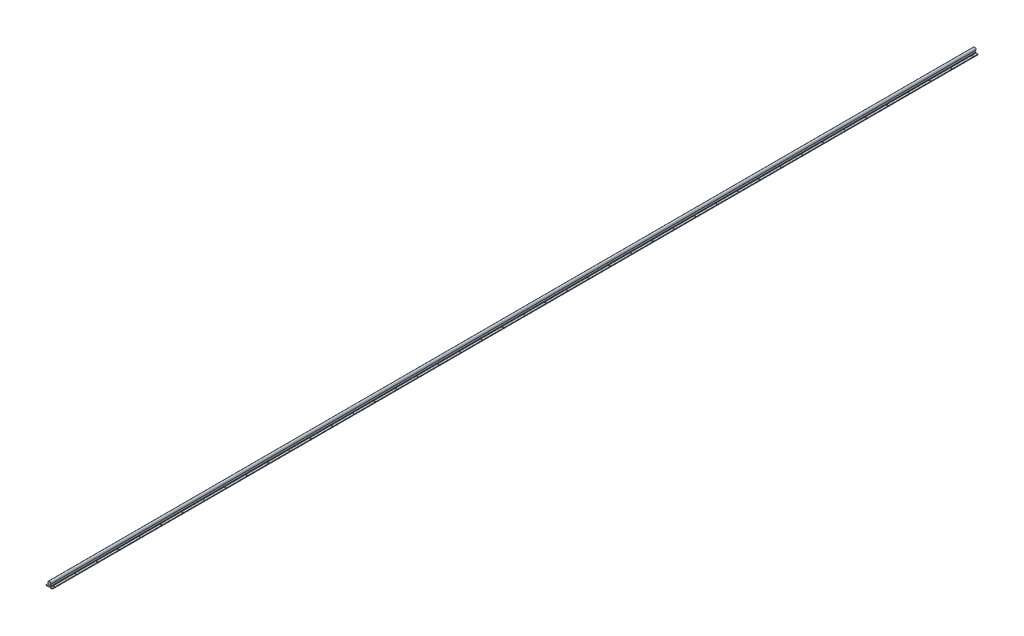
SolidWorks part; units mm, degrees
material "Q235"
ref_plane "Front Plane" through (0, 0, 0) normal (0, 0, 1) x (1, 0, 0)
ref_plane "Top Plane" through (0, 0, 0) normal (0, 1, 0) x (1, 0, 0)
ref_plane "Right Plane" through (0, 0, 0) normal (1, 0, 0) x (0, 0, -1)
sketch "Sketch1" plane through (0, 0, 0) normal (0, 0, 1) x (1, 0, 0)
  line L0 (0, 10) -> (0, -27) construction
  line L1 (4, -9.3) -> (8.4456, -17)
  line L2 (8.4456, -17) -> (9.5, -17)
  line L3 (9.5, -17) -> (9.5, -22)
  line L4 (9.5, -22) -> (22.5, -22)
  line L5 (22.5, -22) -> (22.5, -27)
  line L6 (22.5, -27) -> (0, -27)
  line L7 (-4, -9.3) -> (-8.4456, -17)
  line L8 (15, -22) -> (15, -27) construction
  line L9 (0, -20.5) -> (5.5, -20.5)
  line L10 (5.5, -20.5) -> (5.5, -27)
  line L11 (4, -9.3) -> (4, -9.1652)
  line L12 (-4, -9.3) -> (-4, -9.1652)
  circle A0 centre (0, 0) radius 10
  point P18 (17.75, -22)
  dimension "d" = 20
  dimension "(h)" = 27
  dimension "JD" = 60
  dimension "B" = 45
  dimension "C" = 30
  dimension "T" = 5
  dimension "Y" = 10
  dimension "F" = 19
  dimension "X" = 8
  dimension "a2" = 11
  dimension "a1" = 6.5
  dimension "S1" = 5.5
  dimension "H" = 17.7
sketch "Sketch2" plane through (0, 0, 0) normal (1, 0, 0) x (0, 0, -1)
  line L0 (0, -27) -> (1000, -27) construction
  line L2 (0, -20.5) -> (0, -27) construction
  line L3 (0, 10) -> (0, -27) construction
  line L4 (20, -27) -> (20, 5) construction
  line L5 (23.3, -27) -> (23.3, -9.3)
  line L6 (22.805, 2.195) -> (20, 5)
  line L7 (23.3, -9.3) -> (22.805, -8.805)
  line L8 (22.805, -8.805) -> (22.805, 2.195)
  point P2 (170, -27)
  point P4 (20, -27)
  dimension "D1" = 5
  dimension "N" = 20
  dimension "P" = 150
  dimension "D2" = 135
  dimension "(d1)" = 6.6
  dimension "D3" = 5.61
  dimension "ZL" = 1000
sketch "Sketch3" plane through (0, 0, 0) normal (0, 0, 1) x (1, 0, 0)
  line L0 (0, -20.5) -> (5.5, -20.5) construction
  line L1 (5.5, -20.5) -> (5.5, -27) construction
  line L2 (-4, -9.3) -> (-8.4456, -17) construction
  line L3 (4, -9.3) -> (8.4456, -17) construction
  line L4 (8.4456, -17) -> (9.5, -17) construction
  line L5 (9.5, -17) -> (9.5, -22) construction
  line L6 (9.5, -22) -> (22.5, -22) construction
  line L7 (22.5, -22) -> (22.5, -27) construction
  line L8 (22.5, -27) -> (0, -27) construction
  line L9 (-5.5, -20.5) -> (5.5, -20.5)
  line L10 (5.5, -20.5) -> (5.5, -27)
  line L11 (-4, -9.3) -> (-8.4456, -17)
  line L12 (4, -9.3) -> (8.4456, -17)
  line L13 (8.4456, -17) -> (9.5, -17)
  line L14 (9.5, -17) -> (9.5, -22)
  line L15 (9.5, -22) -> (22.5, -22)
  line L16 (22.5, -22) -> (22.5, -27)
  line L17 (22.5, -27) -> (5.5, -27)
  line L18 (0, 10) -> (0, -27) construction
  line L19 (0, 10) -> (0, -27) construction
  line L20 (-8.4456, -17) -> (-9.5, -17)
  line L21 (-22.5, -27) -> (-5.5, -27)
  line L22 (-22.5, -22) -> (-22.5, -27)
  line L23 (-9.5, -22) -> (-22.5, -22)
  line L24 (-9.5, -17) -> (-9.5, -22)
  line L25 (-5.5, -20.5) -> (-5.5, -27)
  line L26 (4, -9.3) -> (4, -9.1652) construction
  line L27 (-4, -9.3) -> (-4, -9.1652) construction
  line L28 (4, -9.3) -> (4, -9.1652)
  line L29 (-4, -9.3) -> (-4, -9.1652)
  arc A1 (4, -9.1652) -> (-4, -9.1652) centre (0, 0) ccw
extrude "Boss-Extrude1" add sketch "Sketch3" against normal blind 6500
sketch "Sketch4" plane through (0, 0, 0) normal (1, 0, 0) x (0, 0, -1)
  line L0 (22.805, 2.195) -> (20, 5) construction
  line L1 (22.805, -8.805) -> (22.805, 2.195) construction
  line L2 (23.3, -9.3) -> (22.805, -8.805) construction
  line L3 (23.3, -27) -> (23.3, -9.3) construction
  line L4 (22.805, 2.195) -> (20, 5)
  line L5 (22.805, -8.805) -> (22.805, 2.195)
  line L6 (23.3, -9.3) -> (22.805, -8.805)
  line L7 (23.3, -27) -> (23.3, -9.3)
  line L8 (20, 5) -> (20, -27)
  line L10 (20, -27) -> (23.3, -27)
revolve "Cut-Revolve1" cut sketch "Sketch4" angle 360 about L8
sketch "Sketch5" plane through (0, -22, 0) normal (0, 1, 0) x (1, 0, 0)
  circle A0 centre (15, 20) radius 2.75
  dimension "D1" = 5.5
extrude "Cut-Extrude1" cut sketch "Sketch5" against normal through all
mirror "Mirror1" about plane through (0, 0, 0) normal (1, 0, 0) of "Cut-Extrude1"
pattern_linear "LPattern1" count 44 spacing 150 along (0, 0, -1) of "Cut-Revolve1", "Cut-Extrude1", "Mirror1"
chamfer "Chamfer1" distance 1 angle 45 2 edges at (0, 10, -6500) (0, 10, 0)
